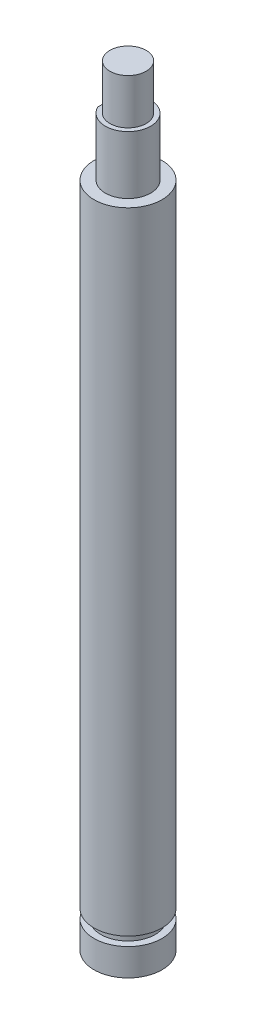
from build123d import *

# Parameters (mm, degrees)
SKETCH2_W          = 3.587001172
SKETCH2_H          = 15.298776085
CUT_EXTRUDE1_DEPTH = 12.8
SKETCH3_W          = 4.275598186
SKETCH3_H          = 2


with BuildPart() as part:
    # Sketch1 → Revolve1 (revolve)
    with BuildSketch(Plane.XY, mode=Mode.PRIVATE) as revolve1_sk:
        Polygon((0, 0), (7.5, 0), (7.5, 147.2), (5, 147.2), (5, 160), (4, 160), (4, 170), (0, 170), align=None)
    revolve(revolve1_sk.sketch.rotate(Axis((0, -11.254736842, 0), (0, 1, 0)), 90), axis=Axis((0, -11.254736842, 0), (0, 1, 0)))

    # Sketch2 → Cut-Extrude1 (cut)
    with BuildSketch(Plane(origin=(0, 160, 0), x_dir=(1, 0, 0), z_dir=(0, 1, 0))):
        with Locations((-6.293500586, -0.885946073)):
            Rectangle(SKETCH2_W, SKETCH2_H)
    extrude(amount=-CUT_EXTRUDE1_DEPTH, mode=Mode.SUBTRACT)

    # Sketch3 → Cut-Revolve1 (revolve, cut)
    with BuildSketch(Plane.XY, mode=Mode.PRIVATE) as cut_revolve1_sk:
        with Locations((8.137799093, 7)):
            Rectangle(SKETCH3_W, SKETCH3_H)
    revolve(cut_revolve1_sk.sketch.rotate(Axis((0, 0, 0), (0, 1, 0)), 90), axis=Axis((0, 0, 0), (0, 1, 0)), mode=Mode.SUBTRACT)


solid = part.part
